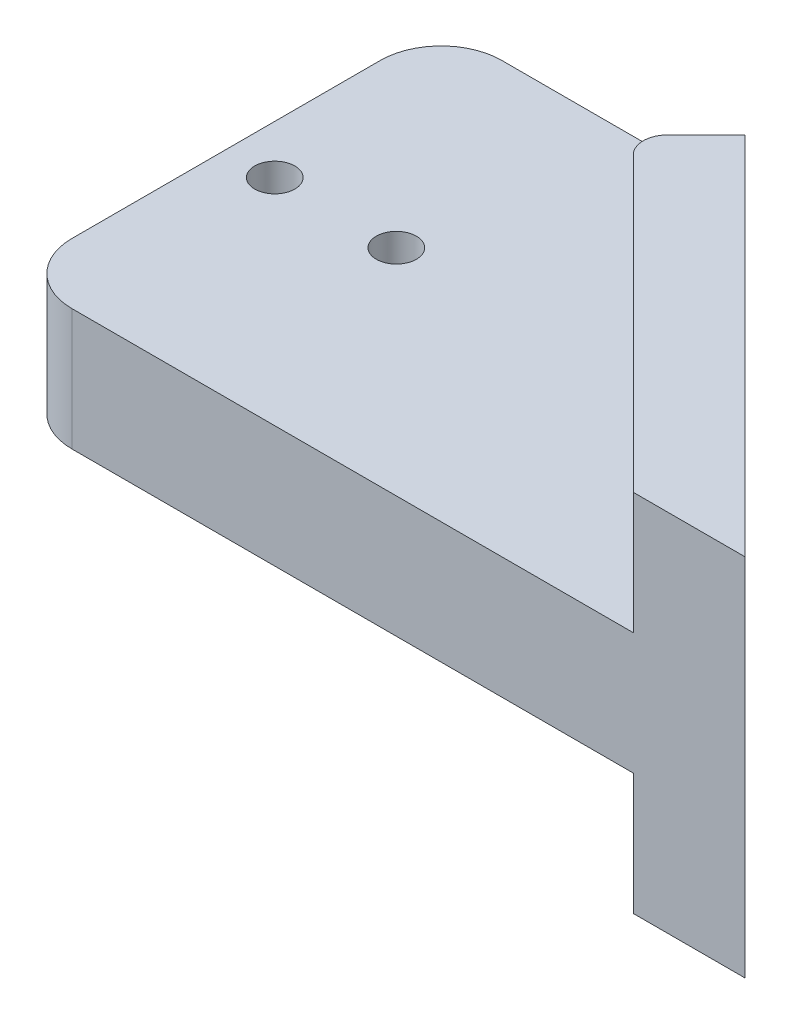
from build123d import *

# Parameters (mm, degrees)
EXTRUDE_1_DEPTH                = 5
HOLE_WIZARD_M4_1_D             = 3.3
EXTRUDE_3_DEPTH                = 10
HOLE_WIZARD_M4_1_2_D           = 4.5
HOLE_WIZARD_M4_1_2_CBORE_D     = 8
HOLE_WIZARD_M4_1_2_CBORE_DEPTH = 4.4
FILLET_1_R                     = 2
FILLET_2_R                     = 5


with BuildPart() as part:
    # 草图1 → 凸台-拉伸1 (new, symmetric)
    with BuildSketch(Plane(origin=(0, 0, 0), x_dir=(1, 0, 0), z_dir=(0, 1, 0))):
        Polygon((-12, -15), (48.355339059, -15), (13, 20.355339059), (-12, 20.355339059), align=None)
    extrude(amount=EXTRUDE_1_DEPTH, both=True)

    # Hole Wizard M4 _1 (through all)
    with Locations(Plane(origin=(0, -5, 0), x_dir=(-1, 0, 0), z_dir=(0, -1, 0))):
        with Locations((8, 2.67766953), (-2, 2.67766953)):
            Hole(HOLE_WIZARD_M4_1_D / 2)

    # 草图5 → 凸台-拉伸3 (add)
    with BuildSketch(Plane.XZ.offset(5)):
        Polygon((13.707106781, -10.455844123), (39.162950904, 15), (48.355339059, 15), (18.303300859, -15.0520382), align=None)
    extrude_3 = extrude(amount=EXTRUDE_3_DEPTH)

    # 镜向1: 凸台-拉伸3 across plane
    add(extrude_3.mirror(Plane.ZX))

    # Hole Wizard M4 _1 2 (through all)
    with Locations(Plane(origin=(12.081475452, 0, -12.081475452), x_dir=(0.7071067811865515, 0, 0.7071067811865436), z_dir=(-0.7071067811865436, 0, 0.7071067811865515))):
        with Locations((8.798989873, 10), (30.798989873, 10), (8.798989873, -10), (30.798989873, -10)):
            CounterBoreHole(HOLE_WIZARD_M4_1_2_D / 2, HOLE_WIZARD_M4_1_2_CBORE_D / 2, HOLE_WIZARD_M4_1_2_CBORE_DEPTH)

    # 圆角1
    fillet_1_edges = [part.edges().sort_by_distance(p)[0] for p in [
        (13.707106781, -10, -10.455844123),
        (13.707106781, 10, -10.455844123),
    ]]
    fillet(fillet_1_edges, radius=FILLET_1_R)

    # 圆角2
    fillet_2_edges = [part.edges().sort_by_distance(p)[0] for p in [
        (-12, 0, 15),
        (-12, 0, -20.355339059),
    ]]
    fillet(fillet_2_edges, radius=FILLET_2_R)


solid = part.part
